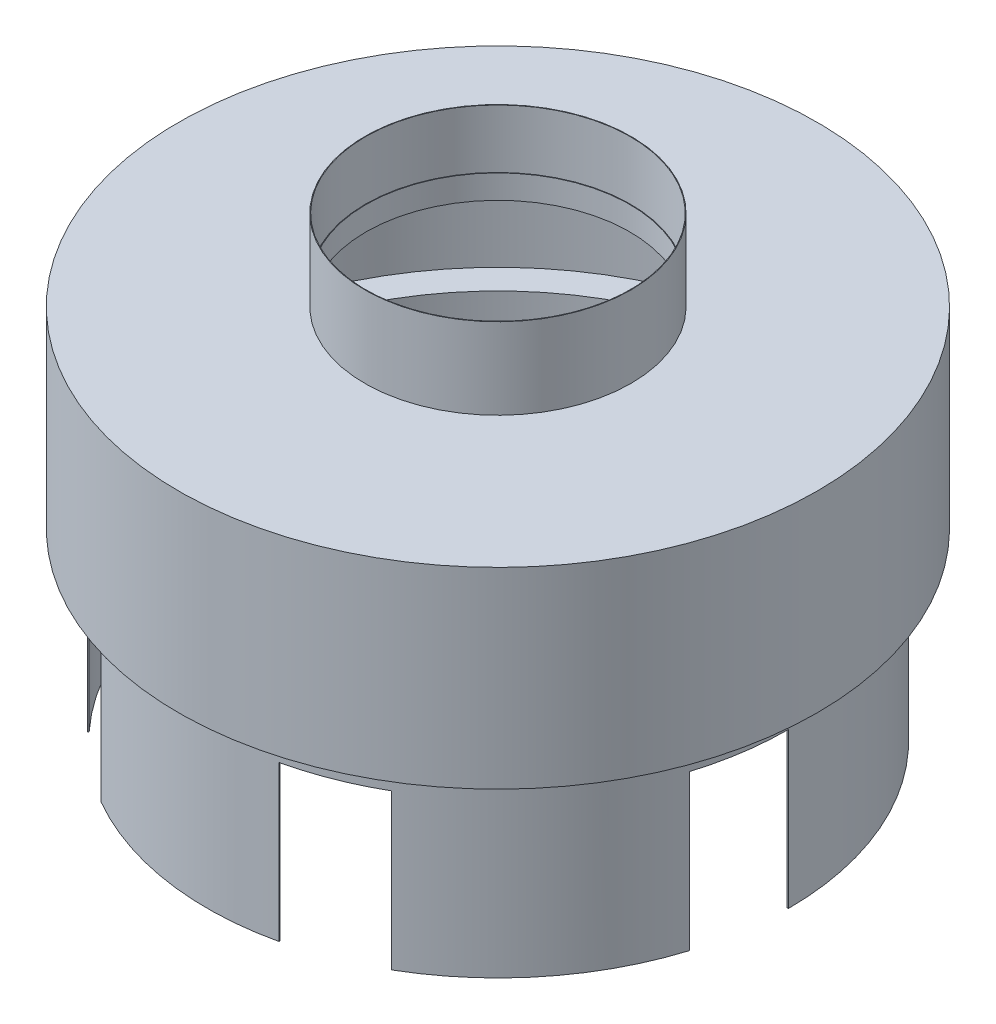
SolidWorks part; units mm, degrees
material "Sheet molding compound plate"
ref_plane "Front Plane" through (0, 0, 0) normal (0, 0, 1) x (1, 0, 0)
ref_plane "Top Plane" through (0, 0, 0) normal (0, 1, 0) x (1, 0, 0)
ref_plane "Right Plane" through (0, 0, 0) normal (1, 0, 0) x (0, 0, -1)
sketch "Sketch1" plane through (0, 0, 0) normal (0, 0, 1) x (1, 0, 0)
  line L0 (0, 0) -> (0, 790)
  line L1 (0, 790) -> (230, 790)
  line L2 (230, 790) -> (230, 650)
  line L3 (230, 650) -> (552, 650)
  line L4 (552, 650) -> (552, 318)
  line L5 (552, 318) -> (502, 318)
  line L6 (502, 318) -> (502, 0)
  line L7 (502, 0) -> (0, 0)
  dimension "D1" = 230
  dimension "D2" = 140
  dimension "D3" = 318
  dimension "D4" = 50
  dimension "D5" = 502
  dimension "D6" = 650
revolve "Revolve1" add sketch "Sketch1" angle 360 about L0
shell "Shell1" thickness 2
sketch "Sketch2" plane through (0, 790, 0) normal (0, 1, 0) x (1, 0, 0)
  circle A3 centre (0, 0) radius 229
  circle A4 centre (0, 0) radius 229
  dimension "D1" = 1
extrude "Cut-Extrude1" cut sketch "Sketch2" against normal blind 101
sketch "Sketch3" plane through (0, 0, 0) normal (0, 1, 0) x (1, 0, 0)
  line L0 (0, 0) -> (635.3842, 0)
  line L3 (0, 0) -> (612.3616, -189.3771)
  line L4 (612.3616, -189.3771) -> (635.3842, 0)
  circle A0 centre (0, 0) radius 502 construction
  point P3 (479.5896, -148.3165)
  point P5 (502, 0)
  dimension "D1" = 150
extrude "Cut-Extrude2" cut sketch "Sketch3" along normal offset from surface (268 mm away) 50 up to face at (552, 318, 0)
pattern_circular "CirPattern1" count 6 over 360 about axis through (0, 0, 0) along (0, 1, 0) of "Cut-Extrude2"
